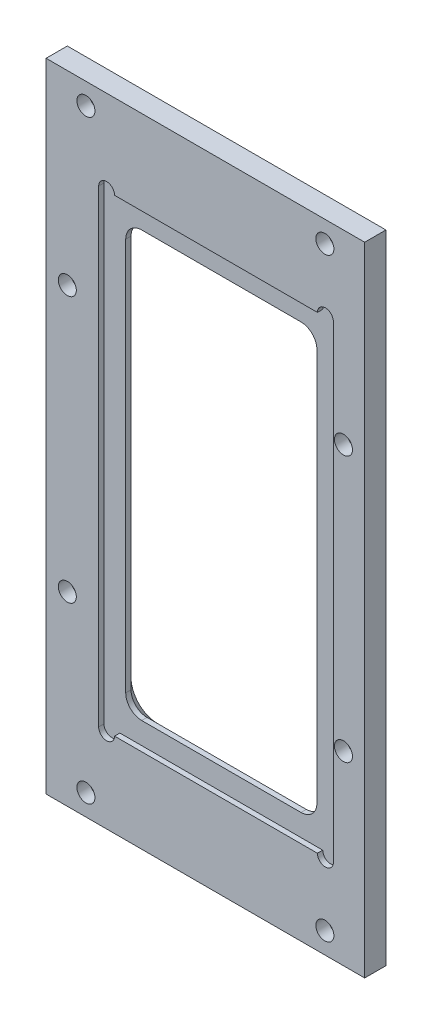
SolidWorks part; units mm, degrees
material "6061Al"
ref_plane "前视基准面" through (0, 0, 0) normal (0, 0, 1) x (1, 0, 0)
ref_plane "上视基准面" through (0, 0, 0) normal (0, 1, 0) x (1, 0, 0)
ref_plane "右视基准面" through (0, 0, 0) normal (1, 0, 0) x (0, 0, -1)
sketch "草图1" plane through (0, 0, 0) normal (0, 0, 1) x (1, 0, 0)
  line L1 (-30, -60) -> (30, -60)
  line L2 (-30, -60) -> (-30, 60)
  line L3 (-30, 60) -> (30, 60)
  line L4 (30, -60) -> (30, 60)
  line L5 (-30, -60) -> (30, 60) construction
  line L6 (-30, 60) -> (30, -60) construction
  point P0 (0, 0)
  dimension "D1" = 120
  dimension "D2" = 60
extrude "凸台-拉伸1" add sketch "草图1" along normal mid plane 4
sketch "草图2" plane through (0, 0, 2) normal (0, 0, 1) x (1, 0, 0)
  line L0 (0, 0) -> (30, 0) construction
  line L1 (30, -60) -> (30, 60) construction
  line L3 (-16, 40) -> (20, 40)
  line L4 (-16, 40) -> (-16, -40)
  line L5 (-16, -40) -> (20, -40)
  line L6 (20, 40) -> (20, -40)
  dimension "D1" = 36
  dimension "D2" = 80
  dimension "D3" = 10
extrude "切除-拉伸1" cut sketch "草图2" against normal through all
sketch "草图3" plane through (0, 0, 2) normal (0, 0, 1) x (1, 0, 0)
  line L8 (24.1, 44.1) -> (-20.1, 44.1)
  line L9 (24.1, -44.1) -> (24.1, 44.1)
  line L10 (-20.1, -44.1) -> (24.1, -44.1)
  line L11 (-20.1, 44.1) -> (-20.1, -44.1)
  line L12 (24.1, 44.1) -> (-20.1, 44.1)
  line L13 (24.1, -44.1) -> (24.1, 44.1)
  line L14 (-20.1, -44.1) -> (24.1, -44.1)
  line L15 (-20.1, 44.1) -> (-20.1, -44.1)
  dimension "D1" = 4.1
extrude "切除-拉伸2" cut sketch "草图3" against normal blind 1
hole_wizard "Ø3.0 (3) 直径孔1" positions "草图4" profile "草图5" hole size "Ø3.0" standard "ISO" end condition up to next
sketch "草图4" plane through (0, 0, 2) normal (0, 0, 1) x (1, 0, 0)
  line L0 (24.1, 44.1) -> (-20.1, 44.1) construction
  line L1 (-20.1, 44.1) -> (-20.1, -44.1) construction
  line L8 (-30, 0) -> (30, 0) construction
  line L9 (-30, 60) -> (-30, -60) construction
  line L10 (30, -60) -> (30, 60) construction
  line L12 (2, 40) -> (2, 73.6475) construction
  line L13 (-16, 40) -> (20, 40) construction
  point P0 (-18.6, 44.1)
  point P17 (22.6, 44.1)
  point P39 (22.6, -44.1)
  point P40 (-18.6, -44.1)
  dimension "D1" = 1.5
sketch "草图5" plane through (-18.6, 44.1, 2) normal (1, 0, 0) x (0, -1, 0)
  line L0 (0, 0) -> (0, 1)
  line L1 (0, 1) -> (1.5, 1)
  line L2 (1.5, 1) -> (1.5, 0)
  line L5 (1.5, 0) -> (0, 0)
  line L11 (0, -6.35) -> (0, 107.95) construction
  dimension "通孔孔直径" = 3
  dimension "通孔孔深度" = 1
fillet "圆角1" radius 3 4 edges at (20, 40, -0.5) (20, -40, -0.5) (-16, -40, -0.5) (-16, 40, -0.5)
chamfer "倒角1" distance 2 angle 45 8 edges at (2, -40, -2) (19.1213, -39.1213, -2) (-15.1213, -39.1213, -2) (20, 0, -2) (-16, 0, -2) (19.1213, 39.1213, -2) (-15.1213, 39.1213, -2) (2, 40, -2)
hole_wizard "M3 六角凹锥坑螺钉的锥形沉头孔1" positions "草图6" profile "草图7" countersink size "M3" standard "ISO" end condition up to next
sketch "草图6" plane through (0, 0, -2) normal (0, 0, -1) x (-1, 0, 0)
  point P0 (-22.5, 56)
  point P3 (22.5, 56)
  point P6 (26, 25)
  point P9 (26, -25)
  point P12 (22.5, -56)
  point P15 (-22.5, -56)
  point P18 (-26, -25)
  point P21 (-26, 25)
sketch "草图7" plane through (22.5, 56, -2) normal (1, 0, 0) x (0, 1, 0)
  line L0 (0, 0) -> (0, 4)
  line L1 (0, 4) -> (1.7, 4)
  line L2 (1.7, 4) -> (1.7, 1.66)
  line L3 (1.7, 1.66) -> (3.36, 0)
  line L5 (3.36, 0) -> (0, 0)
  line L6 (-1.7, 1.66) -> (-3.36, 0) construction
  line L11 (0, -6.35) -> (0, 107.95) construction
  dimension "通孔孔直径" = 3.4
  dimension "通孔孔深度" = 4
  dimension "近端锥形沉头孔直径" = 6.72
  dimension "近端锥形沉头孔角度" = 90
